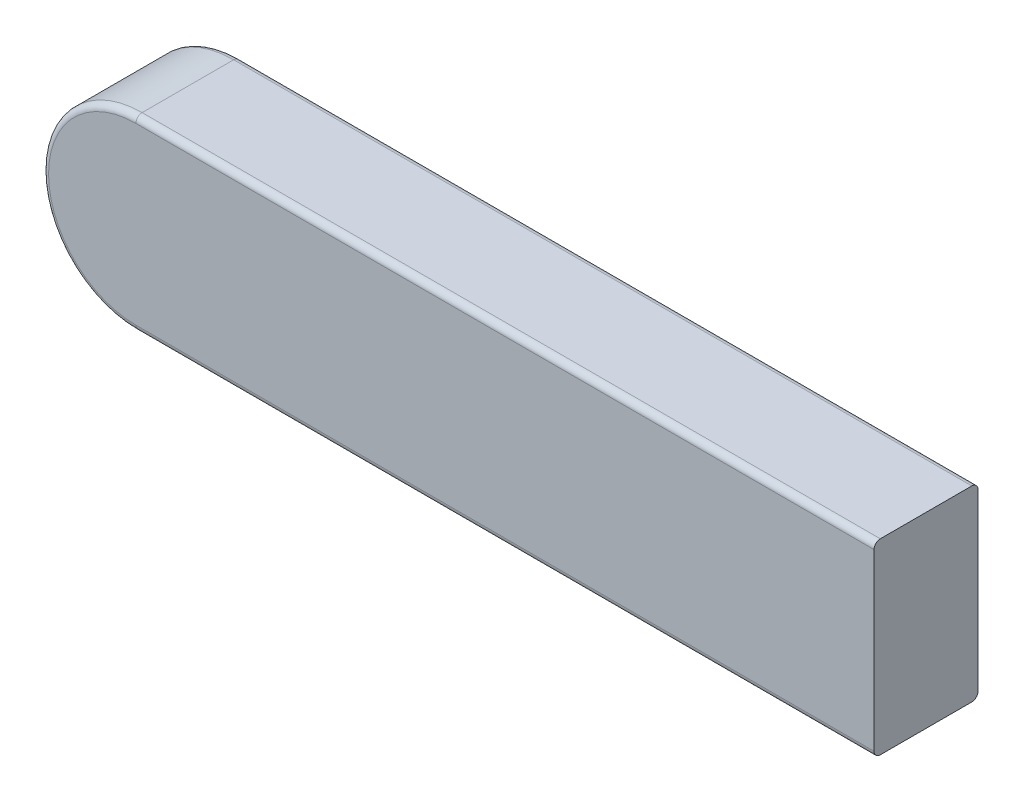
SolidWorks part; units mm, degrees
ref_plane "Plane1" through (0, 0, 0) normal (0, 0, 1) x (1, 0, 0)
ref_plane "Plane2" through (0, 0, 0) normal (0, 1, 0) x (1, 0, 0)
ref_plane "Plane3" through (0, 0, 0) normal (1, 0, 0) x (0, 0, -1)
sketch "Dimension Sketch" plane through (0, 0, 0) normal (0, 0, 1) x (1, 0, 0)
  line L0 (-80, 0) -> (80, 0) construction
  point P3 (-20, 0)
  point P4 (-1.2, 0)
  point P5 (0, 0)
  point P8 (-36, 0)
  point P11 (0, 0)
sketch "Sketch1" plane through (0, 0, 0) normal (0, 0, 1) x (1, 0, 0)
  line L0 (-28.0599, 0) -> (30.562, 0) construction
  line L1 (-9, 18) -> (133, 18)
  line L2 (-9, -18) -> (133, -18)
  line L3 (0, 2.9108) -> (0, -2.1805) construction
  line L4 (133, 18) -> (133, -18)
  arc A0 (-9, 18) -> (-9, -18) centre (-9, 0) ccw
extrude "Base-Extrude" add sketch "Sketch1" along normal blind 20
fillet "Fillet1" radius 1.2 6 edges at (-27, 0, 20) (62, -18, 20) (62, -18, 0) (-27, 0, 0) (62, 18, 0) (62, 18, 20)
equation "\"D3@Sketch1\" = \"L@Dimension Sketch\""
equation "\"D1@Sketch1\" = \"b@Dimension Sketch\" / 2"
equation "\"D1@Fillet1\" = \"r@Dimension Sketch\""
equation "\"D1@Base-Extrude\" = \"h@Dimension Sketch\""
